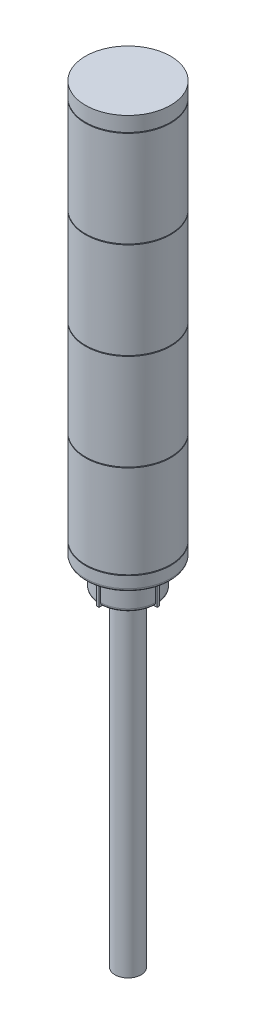
from build123d import *

# Parameters (mm, degrees)
SKETCH_2_W      = 6
SKETCH_2_H      = 0.5
EXTRUDE_1_REACH = 273.501
SKETCH_3_W      = 6
SKETCH_3_H      = 1.5
SKETCH_3_W_2    = 1.5
SKETCH_3_H_2    = 6


with BuildPart() as part:
    # 草图1 → 旋转1 (revolve)
    with BuildSketch(Plane.XY, mode=Mode.PRIVATE) as revolve_1_sk:
        with BuildLine():
            Line((0, 0), (-8, 0))
            Line((-8, 0), (-8, 200))
            Line((-8, 200), (-15.5, 200))
            ThreePointArc((-15.5, 200), (-16.914213562, 200.585786438), (-17.5, 202))
            Line((-17.5, 202), (-17.5, 214))
            ThreePointArc((-17.5, 214), (-17.99058084, 215.312118058), (-19.221653798, 215.980536137))
            Line((-19.221653798, 215.980536137), (-24.278346202, 216.691207909))
            ThreePointArc((-24.278346202, 216.691207909), (-25.50941916, 217.359625988), (-26, 218.671744046))
            Line((-26, 218.671744046), (-26, 469))
            Line((-26, 469), (0, 469))
            Line((0, 469), (0, 0))
        make_face()
    revolve(revolve_1_sk.sketch.rotate(Axis((0, 0, 0), (0, 1, 0)), 270), axis=Axis((0, 0, 0), (0, 1, 0)))

    # 草图2 → 切除-旋转1 (revolve, cut)
    with BuildSketch(Plane.XY, mode=Mode.PRIVATE) as cut_revolve_1_sk:
        with Locations((26, 225.75)):
            Rectangle(SKETCH_2_W, SKETCH_2_H)
        with Locations((26, 282.75)):
            Rectangle(SKETCH_2_W, SKETCH_2_H)
        with Locations((26, 341.75)):
            Rectangle(SKETCH_2_W, SKETCH_2_H)
        with Locations((26, 400.75)):
            Rectangle(SKETCH_2_W, SKETCH_2_H)
        with Locations((26, 459.75)):
            Rectangle(SKETCH_2_W, SKETCH_2_H)
        with Locations((26, 518.75)):
            Rectangle(SKETCH_2_W, SKETCH_2_H)
        with Locations((26, 577.75)):
            Rectangle(SKETCH_2_W, SKETCH_2_H)
    revolve(cut_revolve_1_sk.sketch.rotate(Axis((0, 616.35, 0), (0, -1, 0)), 270), axis=Axis((0, 616.35, 0), (0, -1, 0)), mode=Mode.SUBTRACT)

    # 草图3 → 凸台-拉伸1 (add, up to next)
    with BuildSketch(Plane.XZ.offset(-200), mode=Mode.PRIVATE) as extrude_1_sk1:
        with Locations((15.5, 0)):
            Rectangle(SKETCH_3_W, SKETCH_3_H)
    extrude_1_tool1 = extrude(extrude_1_sk1.sketch, amount=-EXTRUDE_1_REACH, mode=Mode.PRIVATE) - part.part
    # 草图3 → 凸台-拉伸1 (add, up to next)
    with BuildSketch(Plane.XZ.offset(-200), mode=Mode.PRIVATE) as extrude_1_sk2:
        with Locations((0, 15.5)):
            Rectangle(SKETCH_3_W_2, SKETCH_3_H_2)
    extrude_1_tool2 = extrude(extrude_1_sk2.sketch, amount=-EXTRUDE_1_REACH, mode=Mode.PRIVATE) - part.part
    # 草图3 → 凸台-拉伸1 (add, up to next)
    with BuildSketch(Plane.XZ.offset(-200), mode=Mode.PRIVATE) as extrude_1_sk3:
        with Locations((0, -15.5)):
            Rectangle(SKETCH_3_W_2, SKETCH_3_H_2)
    extrude_1_tool3 = extrude(extrude_1_sk3.sketch, amount=-EXTRUDE_1_REACH, mode=Mode.PRIVATE) - part.part
    # 草图3 → 凸台-拉伸1 (add, up to next)
    with BuildSketch(Plane.XZ.offset(-200), mode=Mode.PRIVATE) as extrude_1_sk4:
        with Locations((-15.5, 0)):
            Rectangle(SKETCH_3_W, SKETCH_3_H)
    extrude_1_tool4 = extrude(extrude_1_sk4.sketch, amount=-EXTRUDE_1_REACH, mode=Mode.PRIVATE) - part.part
    add(extrude_1_tool1.solids().sort_by_distance((15.5, 200, 0))[0])
    add(extrude_1_tool2.solids().sort_by_distance((0, 200, 15.5))[0])
    add(extrude_1_tool3.solids().sort_by_distance((0, 200, -15.5))[0])
    add(extrude_1_tool4.solids().sort_by_distance((-15.5, 200, 0))[0])


solid = part.part
